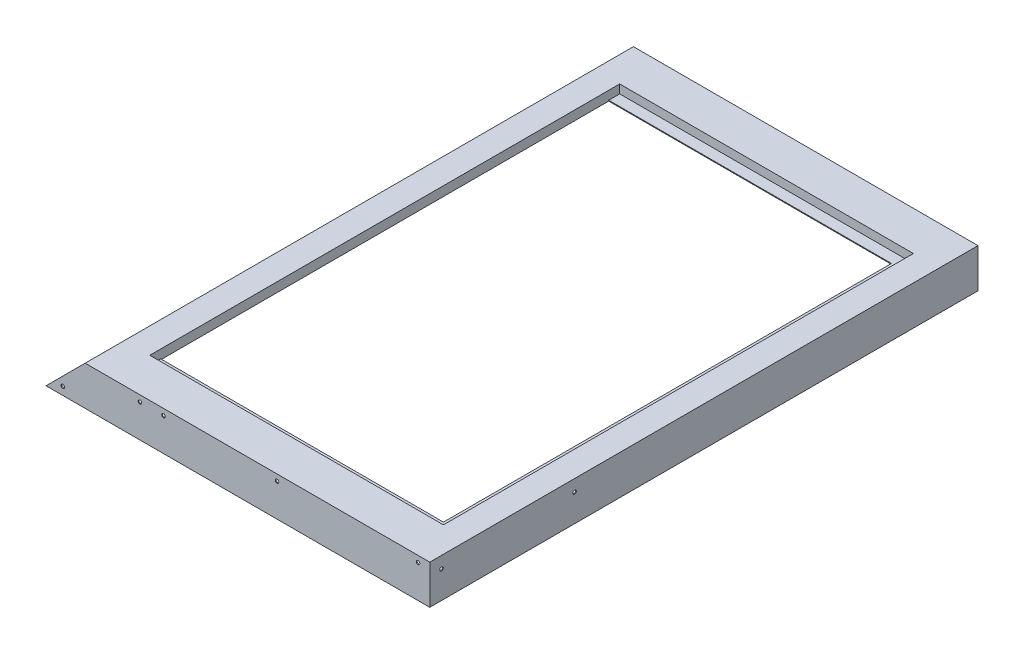
SolidWorks part; units mm, degrees
ref_plane "前视" through (0, 0, 0) normal (0, 0, 1) x (1, 0, 0)
ref_plane "上视" through (0, 0, 0) normal (0, 1, 0) x (1, 0, 0)
ref_plane "右视" through (0, 0, 0) normal (1, 0, 0) x (0, 0, -1)
sketch "草图1" plane through (0, 0, 0) normal (0, 0, 1) x (1, 0, 0)
  line L0 (0, 0) -> (119.2572, 0) construction
  line L1 (0, 0) -> (0, 36.6217) construction
  line L2 (490, 0) -> (460, 0)
  line L3 (490, 0) -> (490, 100)
  line L4 (490, 100) -> (-390, 100)
  line L5 (-390, 100) -> (-490, 0)
  line L6 (460, 0) -> (460, 2)
  line L7 (460, 2) -> (488, 2)
  line L8 (488, 2) -> (488, 98)
  line L9 (488, 98) -> (-389.1716, 98)
  line L10 (-490, 0) -> (-460, 0)
  line L11 (-460, 0) -> (-460, 2)
  line L12 (-460, 2) -> (-485.1716, 2)
  line L13 (-389.1716, 98) -> (-485.1716, 2)
  dimension "D1" = 490
  dimension "D2" = 100
  dimension "D3" = 2
  dimension "D4" = 980
  dimension "D5" = 2
  dimension "D6" = 2
  dimension "D7" = 30
  dimension "D8" = 2
  dimension "D9" = 2
  dimension "D10" = 30
  dimension "D11" = 135
extrude "凸台-拉伸1" add sketch "草图1" along normal mid plane 1400
sketch "草图2" plane through (0, 100, 0) normal (0, 1, 0) x (1, 0, 0)
  line L0 (0, 0) -> (655.667, 0) construction
  line L1 (-50, 0) -> (50, 0) construction
  line L2 (50, 700) -> (50, -238.8498) construction
  line L3 (490, 700) -> (-390, 700) construction
  line L4 (-325, 600) -> (425, 600)
  line L5 (-325, 600) -> (-325, -600)
  line L6 (-325, -600) -> (425, -600)
  line L7 (425, 600) -> (425, -600)
  dimension "D1" = 750
  dimension "D2" = 1200
  dimension "D3" = 600
  dimension "D4" = 375
extrude "切除-拉伸1" cut sketch "草图2" against normal blind 43
sketch "草图3" plane through (0, 100, 0) normal (0, 1, 0) x (1, 0, 0)
  line L0 (50, 700) -> (50, -196.0242) construction
  line L1 (490, 700) -> (-390, 700) construction
  line L2 (490, 0) -> (-139.6954, 0) construction
  line L3 (490, -700) -> (490, 700) construction
  line L4 (-50, 0) -> (50, 0) construction
  line L6 (-325, 600) -> (425, 600)
  line L7 (-325, 600) -> (-325, -600)
  line L8 (-325, -600) -> (425, -600)
  line L9 (425, 600) -> (425, -600)
  line L10 (-327, 602) -> (427, 602)
  line L11 (-327, 602) -> (-327, -602)
  line L12 (-327, -602) -> (427, -602)
  line L13 (427, 602) -> (427, -602)
  dimension "D1" = 1204
  dimension "D2" = 602
  dimension "D3" = 377
  dimension "D4" = 2
extrude "凸台-拉伸2" add sketch "草图3" against normal blind 24
sketch "草图4" plane through (0, 76, 0) normal (0, -1, 0) x (1, 0, 0)
  line L0 (427, 602) -> (427, -602) construction
  line L1 (-327, 602) -> (427, 602)
  line L2 (-327, 602) -> (-327, 572)
  line L3 (-327, 572) -> (397, 572)
  line L4 (427, 602) -> (427, 572)
  line L6 (-327, -602) -> (427, -602)
  line L7 (-327, -602) -> (-327, -572)
  line L8 (-327, -572) -> (397, -572)
  line L9 (427, -602) -> (427, -572)
  line L11 (397, 0) -> (397, 572)
  line L13 (427, -572) -> (427, 572)
  line L14 (397, 0) -> (397, -572)
  dimension "D1" = 30
  dimension "D2" = 30
extrude "凸台-拉伸3" add sketch "草图4" against normal blind 2
sketch "草图5" plane through (0, 0, -700) normal (0, 0, -1) x (-1, 0, 0)
  line L0 (-490, 100) -> (-490, 0)
  line L1 (-490, 0) -> (490, 0)
  line L2 (490, 0) -> (390, 100)
  line L3 (390, 100) -> (-490, 100)
extrude "凸台-拉伸4" add sketch "草图5" against normal blind 2 separate body
sketch "草图6" plane through (0, 0, 0) normal (0, -1, 0) x (1, 0, 0)
  line L0 (460, -700) -> (490, -700) construction
  line L1 (490, -700) -> (-490, -700)
  line L2 (490, -700) -> (490, -670)
  line L3 (490, -670) -> (-490, -670)
  line L4 (-490, -700) -> (-490, -670)
  line L5 (490, -700) -> (-490, -700) construction
  line L6 (-490, 700) -> (-490, -700) construction
  line L7 (490, 700) -> (490, -700) construction
extrude "凸台-拉伸5" add sketch "草图6" against normal blind 2
sketch "草图8" plane through (0, 0, 700) normal (0, 0, 1) x (1, 0, 0)
  line L49 (490, 0) -> (490, 100)
  line L50 (460, 0) -> (490, 0)
  line L51 (-460, 0) -> (460, 0)
  line L52 (-490, 0) -> (-460, 0)
  line L53 (-390, 100) -> (-490, 0)
  line L54 (490, 100) -> (-390, 100)
  line L55 (490, 0) -> (490, 100)
  line L56 (460, 0) -> (490, 0)
  line L57 (-460, 0) -> (460, 0)
  line L58 (-490, 0) -> (-460, 0)
  line L59 (-390, 100) -> (-490, 0)
  line L60 (490, 100) -> (-390, 100)
  dimension "D1" = 0
extrude "凸台-拉伸7" add sketch "草图8" against normal blind 2
sketch "草图9" plane through (0, 0, 698) normal (0, 0, -1) x (-1, 0, 0)
  line L0 (-3.3726, 84) -> (383.3726, 84) construction
  line L1 (389.1716, 98) -> (-488, 98) construction
  line L2 (-490, 0) -> (-490, 100) construction
  line L3 (-488, 98) -> (-488, 2) construction
  line L4 (383.3726, 84) -> (505.6901, -38.3175) construction
  line L5 (485.1716, 2) -> (389.1716, 98) construction
  line L6 (-3.3726, 84) -> (-601.9519, 84) construction
  circle A0 centre (-460, 84) radius 4.5
  circle A1 centre (250, 84) radius 4.5
  circle A2 centre (190, 84) radius 4.5
  circle A3 centre (447.0122, 20.3604) radius 4.5
  circle A4 centre (-100, 84) radius 4.5
  point P19 (437.1716, 50)
  dimension "D2" = 9
  dimension "D3" = 30
  dimension "D4" = 9
  dimension "D5" = 90
  dimension "D6" = 9
  dimension "D7" = 678
  dimension "D9" = 9
  dimension "D10" = 740
  dimension "D11" = 9
  dimension "D12" = 360
  dimension "D1" = 14
  dimension "D8" = 14
extrude "切除-拉伸2" cut sketch "草图9" against normal blind 10
sketch "草图10" plane through (0, 0, -700) normal (0, 0, -1) x (-1, 0, 0)
  line L0 (478.1098, 11.8902) -> (488, 2)
  line L3 (390, 100) -> (488, 2) construction
  line L4 (488, 2) -> (495.0206, -5.0206)
  line L5 (495.0206, -5.0206) -> (488.7813, 5.6951)
  line L6 (488.7813, 5.6951) -> (478.1098, 11.8902)
extrude "切除-拉伸3" cut sketch "草图10" against normal blind 45
sketch "草图11" plane through (0, 0, 0) normal (0, -1, 0) x (1, 0, 0)
  line L0 (490, 0) -> (-656.6209, 0) construction
  line L1 (-460, 698) -> (-460, -670) construction
  line L2 (460, 698) -> (460, -670) construction
  line L3 (490, 700) -> (490, -700) construction
  line L6 (0, -684) -> (0, -58.2841) construction
  line L7 (-490, 700) -> (490, 700) construction
  line L12 (474, 698) -> (474, -684) construction
  line L13 (474, -684) -> (-474, -684) construction
  line L14 (-474, -684) -> (-474, 684) construction
  circle A0 centre (-474, 670) radius 4.5
  circle A1 centre (-474, 0) radius 4.5
  circle A2 centre (-474, -684) radius 4.5
  circle A3 centre (0, -684) radius 4.5
  circle A4 centre (474, -684) radius 4.5
  circle A5 centre (474, 0) radius 4.5
  circle A6 centre (474, 670) radius 4.5
  dimension "D2" = 9
  dimension "D3" = 30
  dimension "D4" = 9
  dimension "D5" = 9
  dimension "D6" = 9
  dimension "D1" = 14
  dimension "D7" = 14
extrude "切除-拉伸4" cut sketch "草图11" against normal blind 5
sketch "草图12" plane through (488, 0, 0) normal (-1, 0, 0) x (0, 0, 1)
  line L1 (700, 0) -> (700, 100) construction
  line L2 (700, 70) -> (-700, 70)
  line L3 (700, 70) -> (-700, 70) construction
  circle A0 centre (670, 70) radius 4.5
  circle A1 centre (330, 70) radius 4.5
  dimension "D2" = 9
  dimension "D3" = 9
  dimension "D4" = 30
  dimension "D5" = 340
  dimension "D1" = 30
extrude "切除-拉伸5" cut sketch "草图12" against normal blind 10
